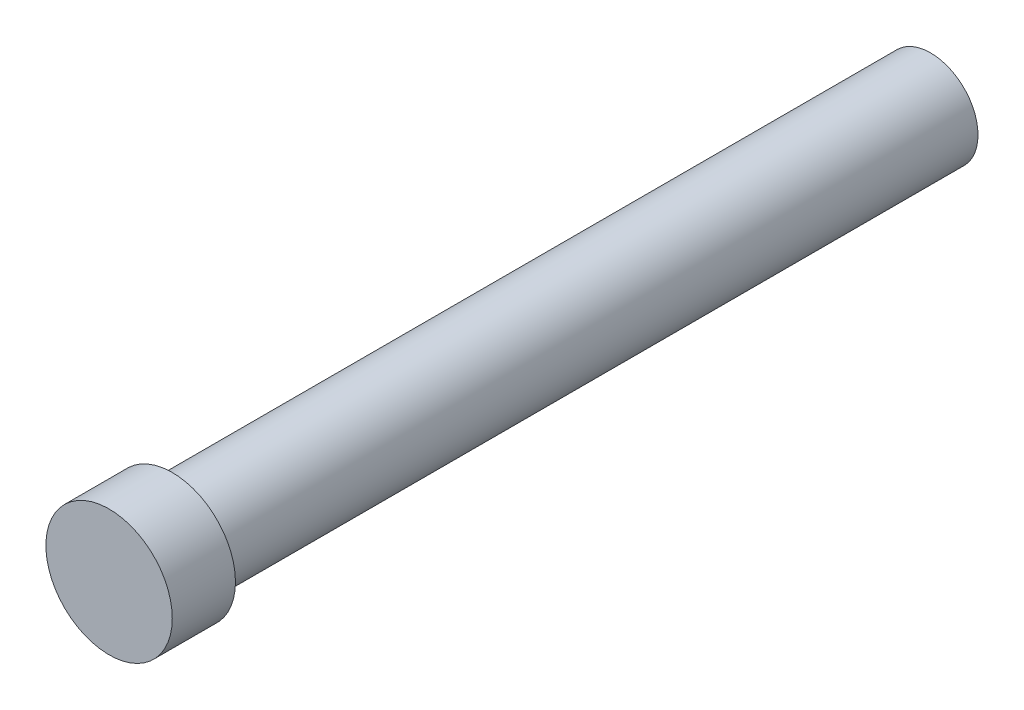
from build123d import *

# Parameters (mm, degrees)
SKETCH_1_R      = 0.75
EXTRUDE_1_DEPTH = 12
SKETCH_2_R      = 1
EXTRUDE_2_DEPTH = 1


with BuildPart() as part:
    # 草图1 → 凸台-拉伸1 (new body)
    with BuildSketch(Plane.XY):
        Circle(SKETCH_1_R)
    extrude(amount=EXTRUDE_1_DEPTH)

    # 草图2 → 凸台-拉伸2 (add)
    with BuildSketch(Plane.XY.offset(12)):
        Circle(SKETCH_2_R)
    extrude(amount=EXTRUDE_2_DEPTH)


solid = part.part
